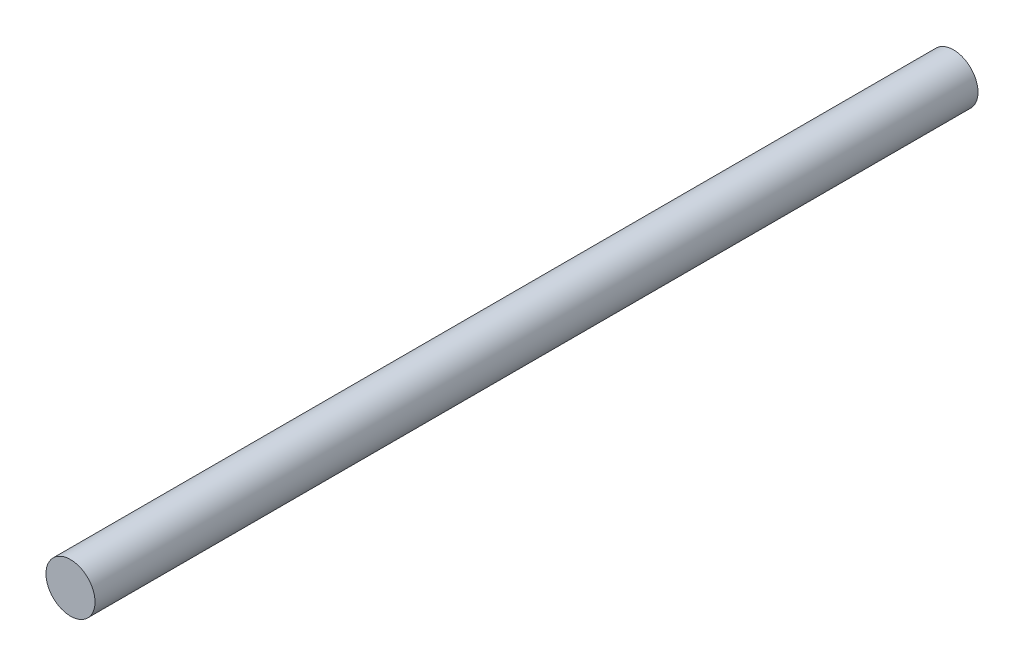
SolidWorks part; units mm, degrees
ref_plane "前视基准面" through (0, 0, 0) normal (0, 0, 1) x (1, 0, 0)
ref_plane "上视基准面" through (0, 0, 0) normal (0, 1, 0) x (1, 0, 0)
ref_plane "右视基准面" through (0, 0, 0) normal (1, 0, 0) x (0, 0, -1)
sketch "草图1" plane through (0, 0, 0) normal (0, 0, 1) x (1, 0, 0)
  circle A0 centre (0, 0) radius 4
  dimension "D1" = 8
extrude "凸台-拉伸1" add sketch "草图1" along normal mid plane 144
